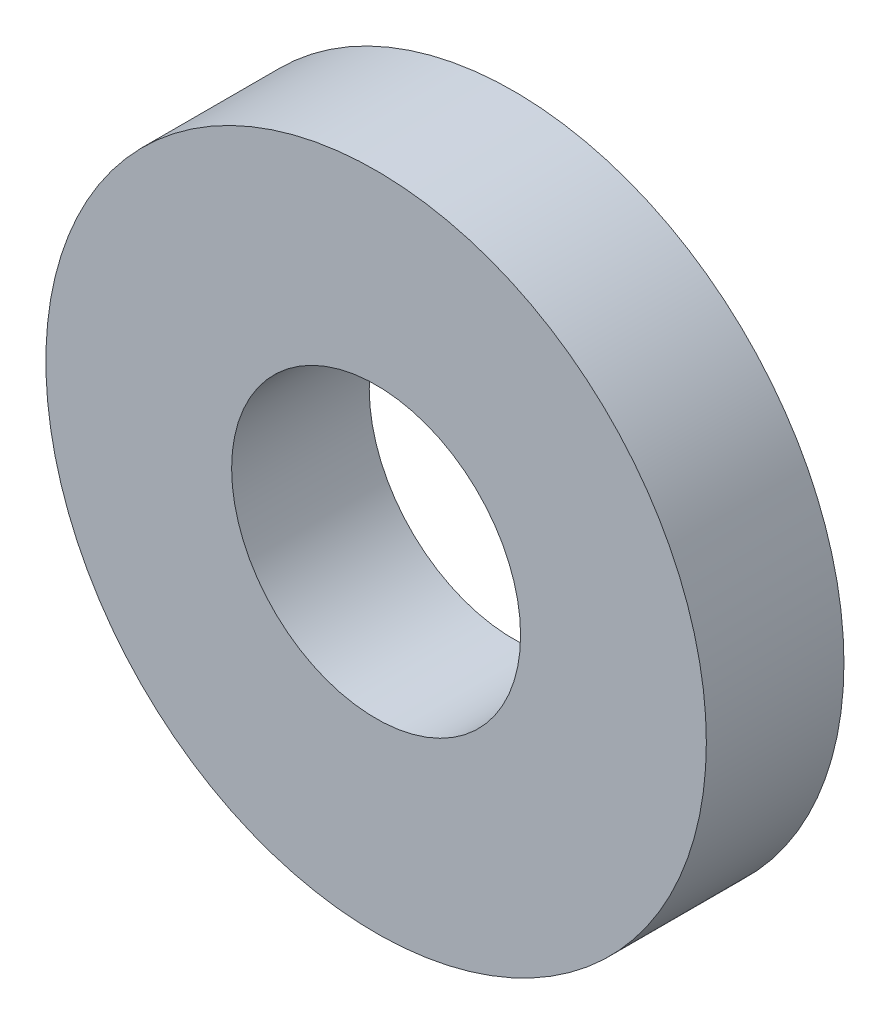
SolidWorks part; units mm, degrees
material "Q235-A"
ref_plane "Front Plane" through (0, 0, 0) normal (0, 0, 1) x (1, 0, 0)
ref_plane "Top Plane" through (0, 0, 0) normal (0, 1, 0) x (1, 0, 0)
ref_plane "Right Plane" through (0, 0, 0) normal (1, 0, 0) x (0, 0, -1)
sketch "Sketch1" plane through (0, 0, 0) normal (0, 0, 1) x (1, 0, 0)
  circle A0 centre (0, 0) radius 12
  circle A1 centre (0, 0) radius 5.25
extrude "Boss-Extrude1" add sketch "Sketch1" along normal blind 5
